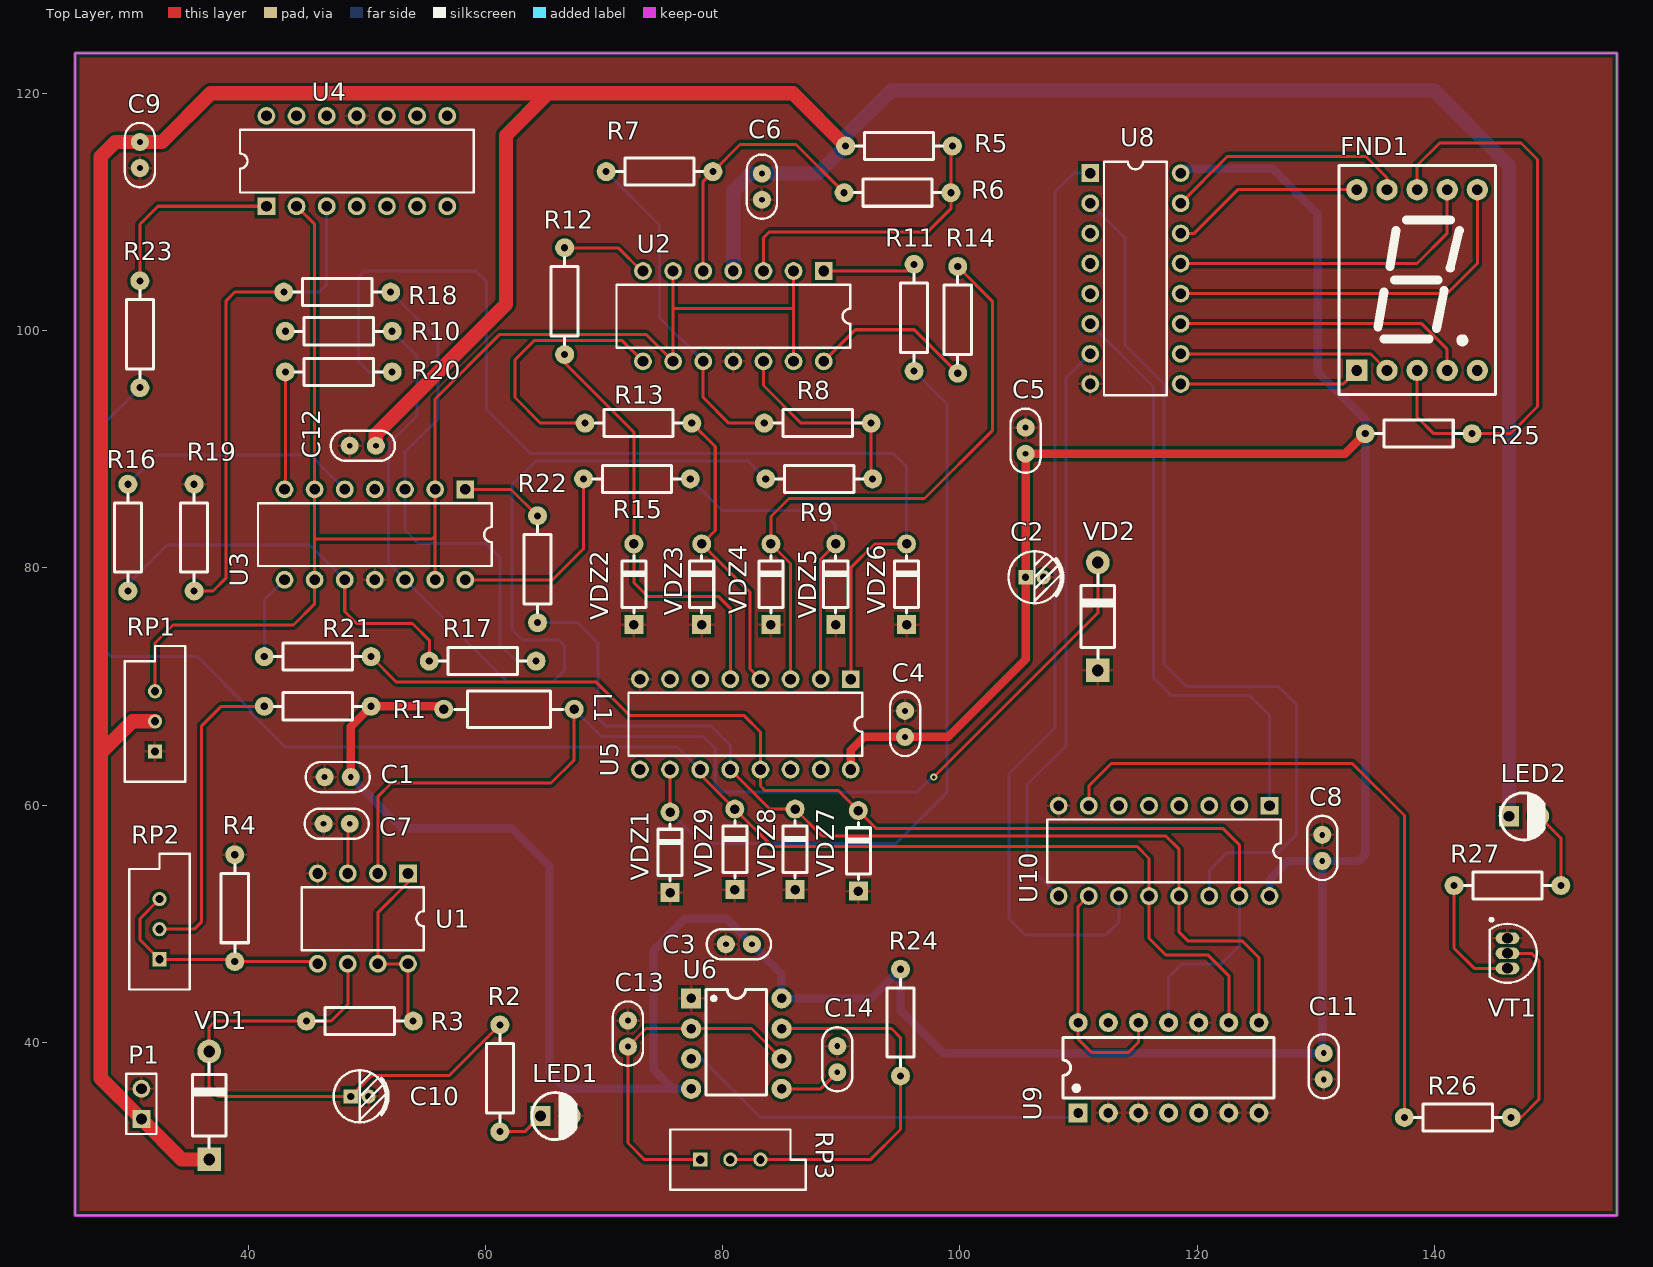
[diagram p0: Top Layer view]
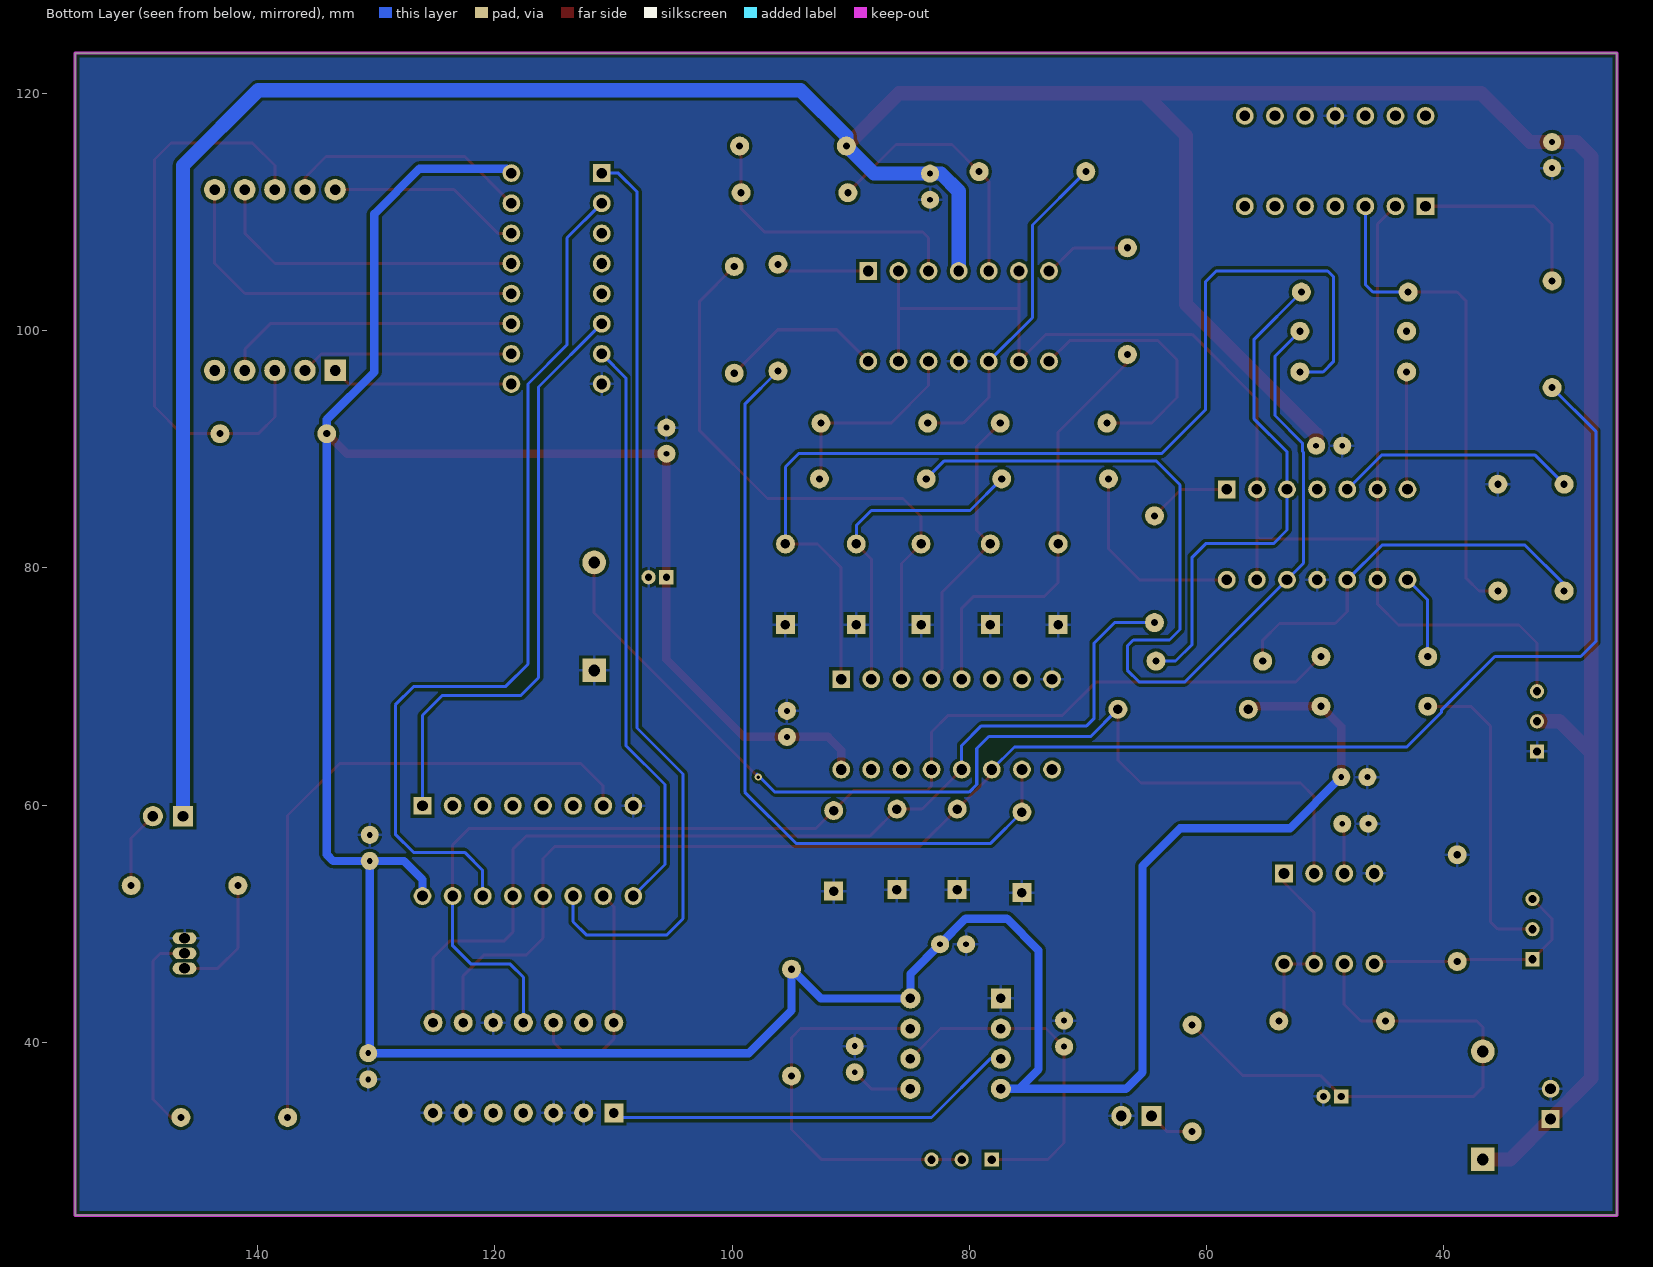
[diagram p1: Bottom Layer view, seen from below]
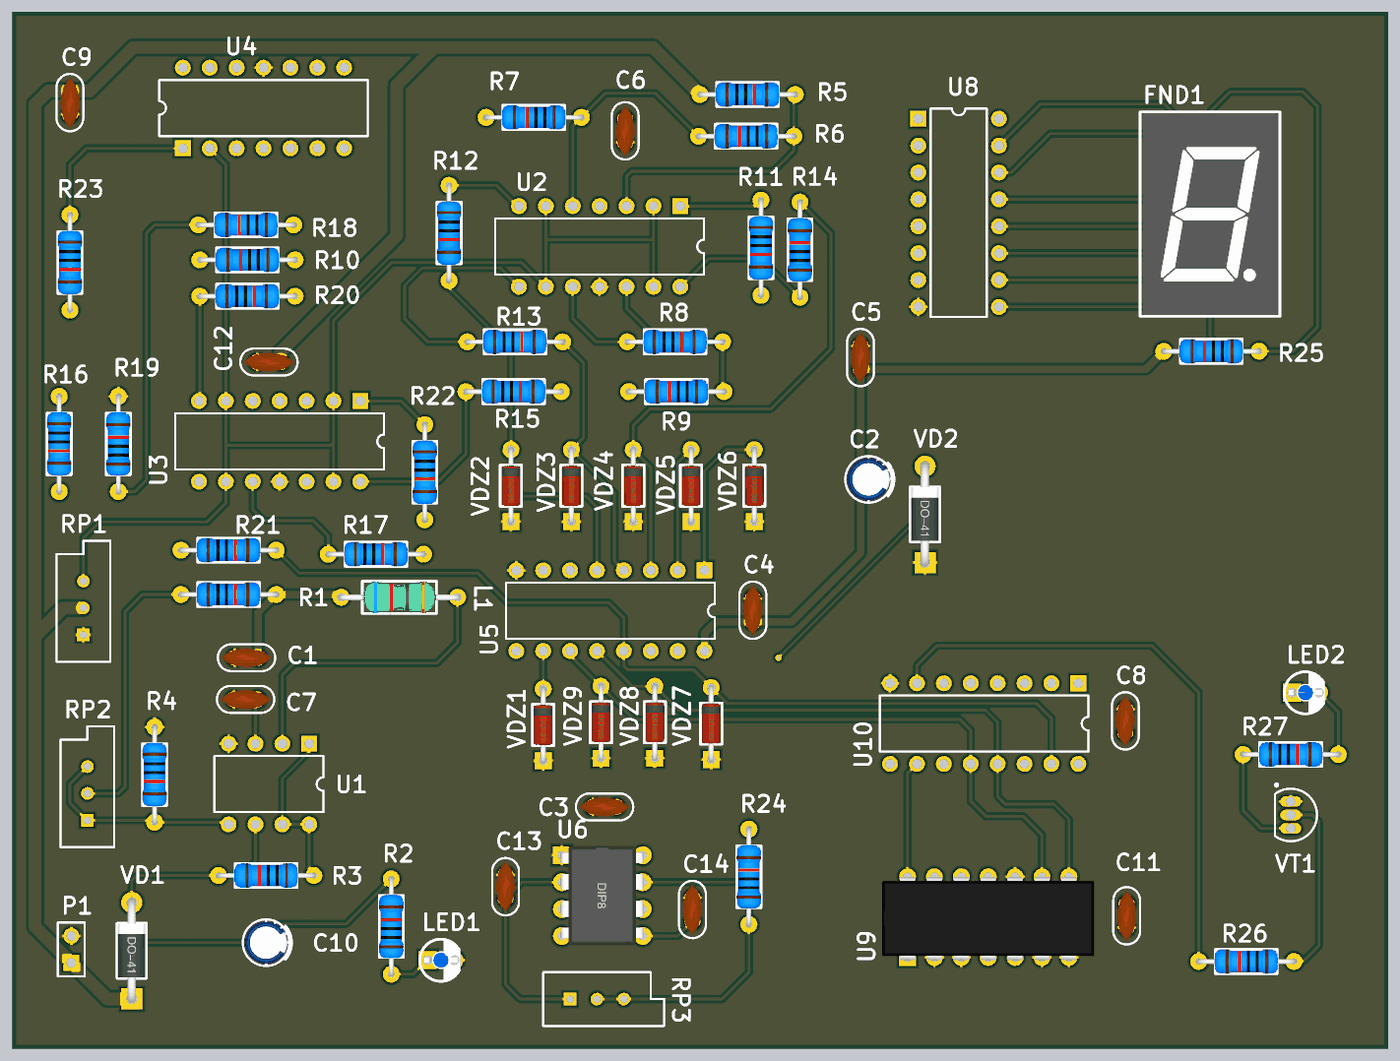
[diagram p2: 3D render of the assembled board from above, using the file's embedded part models]
# Altium PCB MISC80768.PcbDoc
Units mm, origin at the board's own origin, x right, y up, seen from the top; angles counter-clockwise.
Board outline 130 x 98 mm, 2 copper layers (Top Layer, Bottom Layer); 70 components, 65 nets, 254 pads, 1 vias.

## Layer stack, top to bottom (the 12.6 mil dielectric is the usual default, probably not edited)
Top Solder: solder mask 0.0102, Solder Resist, Dk 3.5
Top Layer: signal copper 0.0356
Dielectric 1: dielectric 0.32, FR-4, Dk 4.8
Bottom Layer: signal copper 0.0356
Bottom Solder: solder mask 0.0102, Solder Resist, Dk 3.5

## Board outline
25.4,25.4 25.4,123.4 155.4,123.4 155.4,25.4

## Design rules (kind name [scope] priority, off if disabled: settings)
Clearance [All] p1: gap=0.254
MinimumSolderMaskSliver [All] p1: minsoldermaskwidth=0
PolygonConnect [All] p1: connectstyle=Relief reliefconductorwidth=0.254 reliefentries=4 polygonreliefangle="90 Angle" airgapwidth=0.254
RoutingVias [All] p1: holewidth=0.711 width=1.27 viastyle="Through Hole" minholewidth=0.711 minwidth=1.27 maxholewidth=0.711 maxwidth=1.27
SilkToSilkClearance [All] p1: silktosilkclearance=0
SilkToSolderMaskClearance [IsPad] p1: minsilkscreentomaskgap=0 clearancetoexposedcopper=TRUE
SolderMaskExpansion [All] p1: expansion=0.102
Width [All] p1: maxlimit=2 minlimit=0.254 preferedwidth=0.254
27 further rules are at their usual default settings.

## Components (designator, comment, footprint, x,y, rotation, side; value= is the part's Value field where it differs from the comment)
C1 "104" "CC 2.2*5" 47.541,62.357 r180 top
C2 "470UF" "CAP 1.5*4*8" 106.299,79.205 r0 top
C3 "0.1uF" "CC 2.2*5" 81.364,48.26 r180 top
C4 "0.1uF" "CC 2.2*5" 95.377,66.845 r90 top
C5 "0.1uF" "CC 2.2*5" 105.537,90.721 r90 top
C6 "0.1uF" "CC 2.2*5" 83.312,112.141 r270 top
C7 "470PF" "CC 2.2*5" 47.455,58.42 r180 top
C8 "0.1uF" "CC 2.2*5" 130.556,56.388 r90 top
C9 "0.1uF" "CC 2.2*5" 30.861,114.808 r270 top
C10 "100UF" "CAP 1.5*4*8" 49.391,35.433 r0 top
C11 "0.1uF" "CC 2.2*5" 130.683,37.973 r270 top
C12 "0.1uF" "CC 2.2*5" 49.657,90.297 r180 top
C13 "0.1uF" "CC 2.2*5" 72.009,40.724 r90 top
C14 "0.1uF" "CC 2.2*5" 89.662,38.565 r90 top
FND1 "5011B" "SMG 0.5-1P" 138.557,104.267 r0 top
L1 "220uH" AL0307 61.976,68.072 r0 top
LED1 "red" "LED 3MM-B" 65.913,33.782 r0 top
LED2 "red" "LED 3MM-B" 147.574,59.055 r0 top
P1 "Header 2" HDR1X2 30.988,33.528 r90 top
R1 "3.3K" "RS 1/4W" 45.847,68.326 r0 top
R2 "2.2K" "RS 1/4W" 61.214,36.957 r90 top
R3 "0.5" "RS 1/4W" 49.403,41.783 r180 top
R4 "2.2K" "RS 1/4W" 38.862,51.308 r270 top
R5 "4.7K" "RS 1/4W" 94.869,115.57 r0 top
R6 "4.7K" "RS 1/4W" 94.742,111.633 r180 top
R7 "4.7K" "RS 1/4W" 74.676,113.411 r180 top
R8 "4.7K" "RS 1/4W" 88.011,92.202 r0 top
R9 "4.7K" "RS 1/4W" 88.138,87.503 r180 top
R10 "4.7K" "RS 1/4W" 47.625,99.949 r180 top
R11 "1K" "RS 1/4W" 96.139,101.092 r270 top
R12 "1K" "RS 1/4W" 66.675,102.489 r270 top
R13 "1K" "RS 1/4W" 72.898,92.202 r0 top
R14 "1K" "RS 1/4W" 99.822,100.91 r90 top
R15 "1K" "RS 1/4W" 72.771,87.503 r0 top
R16 "4.7K" "RS 1/4W" 29.845,82.55 r270 top
R17 "4.7K" "RS 1/4W" 59.762,72.136 r0 top
R18 "4.7K" "RS 1/4W" 47.498,103.251 r180 top
R19 "4.7K" "RS 1/4W" 35.433,82.55 r90 top
R20 "1K" "RS 1/4W" 47.625,96.52 r0 top
R21 "1K" "RS 1/4W" 45.847,72.517 r0 top
R22 "1K" "RS 1/4W" 64.389,79.883 r270 top
R23 "1K" "RS 1/4W" 30.861,99.695 r270 top
R24 "20K" "RS 1/4W" 94.996,41.656 r90 top
R25 "330" "RS 1/4W" 138.684,91.313 r180 top
R26 "4.7K" "RS 1/4W" 141.986,33.655 r180 top
R27 "1K" "RS 1/4W" 146.177,53.213 r0 top
RP1 "100K" VR5 32.131,67.056 r90 top
RP2 "5K" VR5 32.512,49.53 r90 top
RP3 "50K" VR5 80.645,30.099 r0 top
U1 "MC34063AP1" 626-05 49.657,50.419 r180 top
U2 "LM324AN" 646-06 80.899,101.219 r180 top
U3 "LM324AN" 646-06 50.673,82.804 r180 top
U4 "LM324AN" 646-06 49.149,114.3 r0 top
U5 "SN74LS147N" 648-08 81.915,66.802 r180 top
U6 "NE555" DIP8 81.153,39.878 r0 top
U8 "SN74LS47N" 648-08 114.808,104.394 r270 top
U9 "SN74LS90" DIP14 109.982,34.036 r90 top
U10 "SN74LS85N" 648-08 117.221,56.134 r180 top
VD1 "1N4007" DO-41 36.703,34.671 r90 top
VD2 "1N5819" DO-41 111.633,75.903 r90 top
VDZ1 "5.1V" DO-35 75.565,56.007 r90 top
VDZ2 "5.1V" DO-35 72.517,78.613 r90 top
VDZ3 "5.1V" DO-35 78.232,78.613 r90 top
VDZ4 "5.1V" DO-35 84.074,78.613 r90 top
VDZ5 "5.1V" DO-35 89.535,78.613 r90 top
VDZ6 "5.1V" DO-35 95.504,78.613 r90 top
VDZ7 "5.1V" DO-35 91.44,56.134 r90 top
VDZ8 "5.1V" DO-35 86.106,56.261 r90 top
VDZ9 "5.1V" DO-35 81.026,56.261 r90 top
VT1 "TP41" TO-92A 146.177,47.498 r180 top

## Footprints (in the part's own frame and the unit in brackets; to place one, negate y for a bottom-side part, rotate by r counter-clockwise, add the part's x,y. Pads: shape width x height; smd on the part's side, far side on the other; paste and mask are expansions set on the pad)
626-05 [mm] "DIP; 8 Leads; Row Spacing 7.62 mm; Pitch 2.54 mm"
  rect 1.5x1.5 hole 0.9: 1(-3.81,-3.81)
  round 1.5 hole 0.9: 2(-1.27,-3.81) 3(1.27,-3.81) 4(3.81,-3.81) 5(3.81,3.81) 6(1.27,3.81) 7(-1.27,3.81) 8(-3.81,3.81)
  silkscreen extent -5.15,-2.65 5.15,2.65
646-06 [mm] "DIP; 14 Leads; Row Spacing 7.62 mm; Pitch 2.54 mm"
  rect 1.5x1.5 hole 0.9: 1(-7.62,-3.81)
  round 1.5 hole 0.9: 2(-5.08,-3.81) 3(-2.54,-3.81) 4(0,-3.81) 5(2.54,-3.81) 6(5.08,-3.81) 7(7.62,-3.81) 8(7.62,3.81) 9(5.08,3.81) 10(2.54,3.81) 11(0,3.81) 12(-2.54,3.81) 13(-5.08,3.81) 14(-7.62,3.81)
  silkscreen extent -9.85,-2.65 9.85,2.65
648-08 [mm] "DIP; 16 Leads; Row Spacing 7.62 mm; Pitch 2.54 mm"
  rect 1.5x1.5 hole 0.9: 1(-8.89,-3.81)
  round 1.5 hole 0.9: 2(-6.35,-3.81) 3(-3.81,-3.81) 4(-1.27,-3.81) 5(1.27,-3.81) 6(3.81,-3.81) 7(6.35,-3.81) 8(8.89,-3.81) 9(8.89,3.81) 10(6.35,3.81) 11(3.81,3.81) 12(1.27,3.81) 13(-1.27,3.81) 14(-3.81,3.81) 15(-6.35,3.81) 16(-8.89,3.81)
  silkscreen extent -9.85,-2.65 9.85,2.65
AL0307 [mm] "11*3*7mm（脚距，直径，长度）"
  round 1.6 hole 0.8: 1(-5.5,0) 2(5.5,0)
  silkscreen extent -4.57,-1.52 4.57,1.52, body extent -5.78,-1.51 5.78,1.51, height 3.06
"CAP 1.5*4*8" [mm] "脚距1.5mm直径4mm高度8mm"
  rect 1.2x1.2 hole 0.6: 1(-0.75,0)
  round 1.2 hole 0.6: 2(0.75,0)
  silkscreen extent -2.2,-2.2 2.41,2.2, body extent -2,-2 2.02,2, height 8.04
"CC 2.2*5" [mm] "脚距2.2mm直径5mm"
  round 1.524 hole 0.5: 1(-1.1,0) 2(1.1,0)
  silkscreen extent -2.71,-1.27 2.71,1.27, body extent -2.4,-0.92 2.4,0.92, height 4.8
DIP8 [mm]
  rect 1.7x1.7 hole 0.8: 1(-3.81,3.81)
  round 1.7 hole 0.8: 2(-3.81,1.27) 3(-3.81,-1.27) 4(-3.81,-3.81) 5(3.81,-3.81) 6(3.81,-1.27) 7(3.81,1.27) 8(3.81,3.81)
  silkscreen extent -2.54,-4.32 2.54,4.57, body extent -3.94,-4.7 3.91,4.7, height 4.5
DIP14 [mm]
  rect 1.6x1.6 hole 0.813: 1(0,0)
  round 1.6 hole 0.813: 2(0,-2.54) 3(0,-5.08) 4(0,-7.62) 5(0,-10.16) 6(0,-12.7) 7(0,-15.24) 8(7.62,-15.24) 9(7.62,-12.7) 10(7.62,-10.16) 11(7.62,-7.62) 12(7.62,-5.08) 13(7.62,-2.54) 14(7.62,0)
  silkscreen extent 1.27,-16.51 6.35,1.27, body extent -0.25,-17.62 7.62,2.38, height 5.1
DO-35 [mm] "1.8*6.8mm(直径，脚距）"
  rect 1.6x1.6 hole 0.8: 1(-3.4,0)
  round 1.6 hole 0.8: 2(3.4,0)
  silkscreen extent -2.41,-1.02 2.41,1.02, body extent -3.65,-0.9 3.65,0.9, height 1.85
DO-41 [mm] "2.6*9.1mm(直径，脚距）"
  rect 2x2 hole 1: 1(-4.55,0)
  round 2 hole 1: 2(4.55,0)
  silkscreen extent -3.56,-1.4 3.56,1.4, body extent -4.92,-1.29 4.98,1.31, height 2.65
HDR1X2 [mm] "Connector; Header; 2 Position"
  rect 1.5x1.5 hole 0.9: 1(0,0)
  round 1.5 hole 0.9: 2(2.54,0)
  silkscreen extent -1.27,-1.27 3.81,1.27
"LED 3MM-B" [mm]
  rect 1.7x1.7 hole 0.9: 1(-1.27,0)
  round 1.7 hole 0.9: 2(1.27,0)
  silkscreen extent -2.01,-2 1.72,1.98, body extent -1.95,-1.95 1.64,1.95, height 5.55
"RS 1/4W" [mm] "直插色环电阻，脚距9mm，直径2.3mm"
  round 1.6 hole 0.6: 1(-4.5,0) 2(4.5,0)
  silkscreen extent -3.68,-1.14 3.68,1.14, body extent -4.72,-1.16 4.73,1.16, height 2.32
"SMG 0.5-1P" [mm] "12.7*19*8mm(长宽厚)"
  rect 1.8x1.8 hole 0.9: 1(-5.08,-7.62)
  round 1.8 hole 0.9: 2(-2.54,-7.62) 3(0,-7.62) 4(2.54,-7.62) 5(5.08,-7.62) 6(5.08,7.62) 7(2.54,7.62) 8(0,7.62) 9(-2.54,7.62) 10(-5.08,7.62)
  silkscreen extent -6.6,-9.65 6.6,9.65, body extent -6.35,-9.5 6.35,9.5, height 8
TO-92A [mm] "TO, Flat Index; 3 In-Line, Axial Leads; Body Dia. 4.5mm; Leads 0.51 x 0.48 mm (max)"
  oval 2x1 hole 0.9: 1(0,-1.27) 2(0,0) 3(0,1.27)
  silkscreen extent -2.48,-2.95 1.5,2.48, body extent -2.48,-2.5 1.5,2.5, height 6.86
VR5 [mm] "Thru-Hole; 3 Leads"
  rect 1.2x1.2 hole 0.7: 1(-2.54,0)
  round 1.2 hole 0.7: 2(0,0) 3(2.54,0)
  silkscreen extent -5.08,-2.54 6.35,2.54

## Part data
C1 C3 C4 C5 C6 C7 C8 C9 C11 C12 C13 C14: library part CC, "ceramic capacitor"
C2 C10: library part "Cap Pol2", "Polarized Capacitor (Axial)"
FND1: "0.5 inch 1-digit common-anode seven-segment display"
L1: library part L-AL, "color-band inductor"
LED1 LED2: library part LED-3MM, "3mm through-hole LED"
P1: "Header, 2-Pin"
R1 R2 R3 R4 R5 R6 R7 R8 R9 R10 R11 R12 R13 R14 R15 R16 R17 R18 R19 R20 R21 R22 R23 R24 R25 R26 R27: library part R-S, "color-band resistor"
RP1 RP2 RP3: library part RPot, "Potentiometer"
U1: "DC-to-DC Converter Control Circuit"
U2 U3 U4: "Quad Low-Power Operational Amplifier"
U5: "10-Line-to-4-Line Priority Encoder"
U6: library part NE555D, "General-Purpose Single Bipolar Timer"
U8: "BCD to 7-Segment Decoder/Driver"
U9: "DECADE DIV-BY-12 BIN CNT"
U10: "4-Bit Magnitude Comparator"
VD1: "rectifier diode"
VD2: library part 1N4007, "rectifier diode"
VDZ1 VDZ2 VDZ3 VDZ4 VDZ5 VDZ6 VDZ7 VDZ8 VDZ9: library part 1N4619, "3V/0.5W zener diode"
VT1: library part 2N3904, "NPN General Purpose Amplifier"

## Via types
v1: diameter 0.61, hole 0.305, Top Layer to Bottom Layer, 1 vias

## Nets (pads, with @x,y where several pads share a name; then routed paths per layer and width w, separated by ;. In a path a pad name is that pad's centre, name@x,y a point inside that pad or via, vN(x,y) a via of type N, cw(c..) or ccw(c..) an arc to the next point about the centre after c; other vN are vias at no path point)
+5V: C1.1 C2.1 C3.1 C4.1 C5.1 C8.1 C11.1 L1.1 R1.2 R24.2 R25.2 U5.16 U6.4 U6.8 U8.16 U10.16 | length 304.5
  Top Layer w0.7: C1.1 48.641,66.62 R1.2 56.222,68.326 L1.1 ; U5.16 90.805,64.643 91.907,65.745 C4.1 99.019,65.745 105.549,72.275 C2.1 105.549,89.609 C5.1 132.492,89.621 R25.2
  Bottom Layer w0.7: C1.1 52.959,58.039 62.23,58.039 65.405,54.864 65.405,37.465 66.802,36.068 75.819,36.068 ; U6.4 75.819,36.068 ; U8.16 118.999,113.665 126.365,113.665 130.175,109.855 130.175,96.52 134.184,92.511 R25.2 134.184,55.825 133.647,55.288 C8.1 ; U10.16 126.111,53.721 127.678,55.288 C8.1 ; 75.819,36.068 74.168,37.719 74.168,47.752 76.835,50.419 80.305,50.419 C3.1 84.963,45.761 U6.8 92.528,43.688 R24.2 94.996,42.672 98.595,39.073 C11.1 130.556,39.2 C8.1
+10V: C6.1 C9.1 C12.1 LED2.1 P1.1 R5.1 RP1.2 U2.4 VD1.1 | length 331.6
  Top Layer w1.2: RP1.2 30.226,67.056 27.559,64.389 ; VD1.1 34.395,30.121 P1.1 27.559,36.957 27.559,64.389 ; C12.1 50.757,91.27 61.722,102.235 61.722,116.459 65.278,120.015 ; R5.1 85.924,120.015 65.278,120.015 ; 27.559,64.389 27.559,114.681 28.786,115.908 C9.1 32.723,115.908 36.83,120.015 65.278,120.015
  Bottom Layer w1.2: U2.4 80.899,111.76 82.38,113.241 C6.1 88.04,113.241 R5.1 90.369,116.404 94.234,120.269 139.954,120.269 146.304,113.919 LED2.1
A: R10.2
CLK: U6.3 U9.1 | length 34.8
  Bottom Layer w0.254: U6.3 78.232,38.608 83.185,33.655 109.601,33.655 U9.1
D0: U9.12 U9.14 U10.10 | length 20
  Top Layer w0.254: U10.10 109.982,51.435 U9.14 109.982,40.259 111.125,39.116 114.173,39.116 115.062,40.005 U9.12
D1: R23.2 U5.11 U9.9 U10.12 VDZ9.2 | length 138.4
  Top Layer w0.254: U5.11 78.105,62.582 VDZ9.2 84.172,56.515 114.935,56.515 115.951,55.499 U10.12 115.951,48.768 117.348,47.371 120.904,47.371 122.682,45.593 U9.9
  Bottom Layer w0.254: R23.2 27.178,91.512 27.178,73.787 28.448,72.517 35.687,72.517 40.166,68.038 40.166,67.837 43.106,64.897 76.2,64.897 U5.11
D2: R22.2 U5.12 U9.8 U10.13 VDZ8.2 | length 87
  Top Layer w0.254: U5.12 83.976,59.661 VDZ8.2 88.363,57.404 117.348,57.404 118.491,56.261 U10.13 118.491,49.276 119.253,48.514 123.825,48.514 125.222,47.117 U9.8
  Bottom Layer w0.254: R22.2 67.746,75.383 69.469,73.66 69.469,67.31 70.104,66.675 78.994,66.675 80.645,65.024 U5.12
D3: R21.2 U5.13 U9.11 U10.15 VDZ7.2 | length 101.9
  Top Layer w0.254: R21.2 52.506,70.358 69.342,70.358 72.136,67.564 81.788,67.564 83.185,66.167 U5.13 83.185,61.595 83.566,61.214 89.76,61.214 VDZ7.2 92.935,58.039 122.174,58.039 123.571,56.642 U10.15
  Bottom Layer w0.254: U9.11 117.602,45.466 118.745,46.609 122.047,46.609 123.571,48.133 U10.15
D4: R20.2 U5.1 VDZ6.2 | length 91.4
  Top Layer w0.254: U5.1 90.805,80.01 92.808,82.013 VDZ6.2
  Bottom Layer w0.254: R20.2 50.165,96.52 49.276,97.409 49.276,104.521 49.784,105.029 59.182,105.029 60.071,104.14 60.071,93.345 63.754,89.662 94.361,89.662 95.504,88.519 VDZ6.2
D5: R15.2 U5.2 VDZ5.2 | length 27.4
  Top Layer w0.254: U5.2 88.265,80.743 VDZ5.2
  Bottom Layer w0.254: R15.2 79.938,84.836 88.265,84.836 89.535,83.566 VDZ5.2
D6: R14.2 U5.3 VDZ4.2 | length 51.1
  Top Layer w0.254: U5.3 85.725,80.362 VDZ4.2 84.074,84.328 85.598,85.852 97.028,85.852 102.743,91.567 102.743,102.489 R14.2
D7: R13.2 U5.4 VDZ3.2 | length 24.9
  Top Layer w0.254: R13.2 79.375,90.225 79.375,83.156 VDZ3.2 82.296,77.949 82.296,71.501 U5.4
D8: R12.2 U5.5 VDZ2.2 | length 36.7
  Top Layer w0.254: R12.2 66.675,97.282 72.517,91.44 VDZ2.2 72.517,78.74 73.66,77.597 79.629,77.597 80.645,76.581 U5.5
D9: R11.2 U5.10 VDZ1.2 | length 66.5
  Top Layer w0.254: VDZ1.2 U5.10
  Bottom Layer w0.254: VDZ1.2 78.203,56.769 94.615,56.769 98.933,61.087 98.933,93.798 R11.2
DQ0: U8.7 U10.9 | length 49
  Bottom Layer w0.254: U10.9 105.664,54.991 105.664,61.722 108.966,65.024 108.966,96.012 U8.7
DQ1: U8.1 U10.11 | length 79
  Bottom Layer w0.254: U8.1 109.601,113.284 108.03,111.713 108.03,66.501 104.14,62.611 104.14,50.419 105.537,49.022 112.268,49.022 113.411,50.165 U10.11
DQ2: U8.2 U10.14 | length 75.7
  Bottom Layer w0.254: U8.2 113.919,107.823 113.919,98.806 117.221,95.504 117.221,71.882 119.126,69.977 126.873,69.977 128.397,68.453 128.397,57.531 126.873,56.007 122.555,56.007 121.031,54.483 U10.14
DQ3: U8.6 U10.1 | length 50.8
  Bottom Layer w0.254: U8.6 116.332,95.25 116.332,70.739 117.856,69.215 124.46,69.215 126.111,67.564 U10.1
GND: C1.2 C2.2 C3.2 C4.2 C5.2 C6.2 C7.2 C8.2 C9.2 C10.2 C11.2 C12.2 C13.2 C14.2 LED1.2 P1.2 R4.1 R19.2 RP1.1 U1.4 U2.11 U3.11 U4.11 U5.8 U6.1 U8.8 U9.2 U9.3 U9.6 U9.7 U9.10 U10.8 VD2.1 VDZ1.1 VDZ2.1 VDZ3.1 VDZ4.1 VDZ5.1 VDZ6.1 VDZ7.1 VDZ8.1 VDZ9.1 VT1.1
NetC7_1: C7.1 U1.3 | length 4.3
  Top Layer w0.254: U1.3 48.387,58.252 C7.1
NetC10_1: C10.1 R2.2 R3.2 U1.6 VD1.2 | length 48.3
  Top Layer w0.254: U1.6 48.387,43.18 46.99,41.783 R3.2 37.211,41.783 36.703,41.275 VD1.2 36.703,36.195 37.465,35.433 C10.1 50.419,37.211 56.968,37.211 R2.2
NetC13_1: C13.1 RP3.1 U6.2 U6.6 | length 29.4
  Top Layer w0.254: RP3.1 73.406,30.099 72.009,31.496 C13.1 73.533,41.148 U6.2 82.423,41.148 U6.6
NetC14_1: C14.1 U6.5 | length 5.3
  Top Layer w0.254: U6.5 88.265,36.068 C14.1
NetFND1_1: FND1.1 U8.9 | length 15.3
  Top Layer w0.254: U8.9 132.334,95.504 FND1.1
NetFND1_2: FND1.2 U8.10 | length 18
  Top Layer w0.254: U8.10 134.62,98.044 FND1.2
NetFND1_3: FND1.3 FND1.8 R25.1 | length 50
  Top Layer w0.254: FND1.3 138.557,92.71 139.954,91.313 R25.1 146.431,91.313 148.717,93.599 148.717,114.427 147.32,115.824 140.462,115.824 138.557,113.919 FND1.8
NetFND1_4: FND1.4 U8.11 | length 25.2
  Top Layer w0.254: U8.11 138.938,100.584 141.097,98.425 FND1.4
NetFND1_6: FND1.6 U8.12 | length 32.3
  Top Layer w0.254: U8.12 141.097,103.124 143.637,105.664 FND1.6
NetFND1_7: FND1.7 U8.13 | length 27.2
  Top Layer w0.254: U8.13 138.557,105.664 141.097,108.204 FND1.7
NetFND1_9: FND1.9 U8.15 | length 20.8
  Top Layer w0.254: U8.15 122.555,114.681 134.239,114.681 136.017,112.903 FND1.9
NetFND1_10: FND1.10 U8.14 | length 16.4
  Top Layer w0.254: U8.14 119.761,108.204 123.444,111.887 FND1.10
NetL1_2: L1.2 U1.2 VD2.2 | length 88.2
  Top Layer w0.254: U1.2 50.927,60.706 52.07,61.849 65.532,61.849 67.476,63.793 L1.2 ; v1(97.79,62.357) 111.633,76.2 VD2.2
  Bottom Layer w0.254: L1.2 69.762,65.786 78.359,65.786 79.375,64.77 79.375,61.722 80.01,61.087 96.393,61.087 v1@97.917,62.611
NetLED1_1: LED1.1 R2.1 | length 4
  Top Layer w0.254: R2.1 63.318,32.457 LED1.1
NetLED2_2: LED2.2 R27.2 | length 6.6
  Top Layer w0.254: LED2.2 150.677,57.222 R27.2
NetR1_1: R1.1 RP2.2 | length 26.3
  Top Layer w0.254: RP2.2 35.433,49.53 36.068,50.165 36.068,66.675 37.719,68.326 R1.1
NetR3_1: R3.1 U1.1 U1.7 U1.8 | length 16.2
  Top Layer w0.254: U1.1 53.467,53.467 50.927,50.927 U1.7 U1.8 53.467,42.219 R3.1
NetR4_2: R4.2 RP2.1 RP2.3 U1.5 | length 19.9
  Top Layer w0.254: RP2.3 30.861,50.419 30.861,48.641 RP2.1 38.68,46.99 R4.2 45.648,46.808 U1.5
NetR5_2: R5.2 R6.1 U2.3 | length 25
  Top Layer w0.254: U2.3 83.439,107.823 83.947,108.331 97.282,108.331 99.242,110.291 R6.1 99.242,115.443 R5.2
NetR6_2: R6.2 R7.1 U2.5 | length 22.4
  Top Layer w0.254: U2.5 78.359,112.594 R7.1 81.462,115.697 86.178,115.697 R6.2
NetR7_2: R7.2 R8.1 U2.10 | length 28.5
  Top Layer w0.254: U2.10 78.359,94.361 80.518,92.202 R8.1
  Bottom Layer w0.254: R7.2 74.676,108.911 74.676,101.092 U2.10
NetR8_2: R8.2 R9.1 U2.12 | length 17.2
  Top Layer w0.254: U2.12 83.439,95.377 86.614,92.202 R8.2 92.511,87.63 R9.1
NetR9_2: R9.2 R10.1 U3.12 | length 83
  Bottom Layer w0.254: R10.1 54.229,97.845 54.229,92.837 51.9,90.508 51.9,89.824 51.816,89.74 51.816,80.391 U3.12 61.849,70.358 65.659,70.358 66.675,71.374 66.675,73.406 66.167,73.914 63.119,73.914 62.23,74.803 62.23,86.995 64.262,89.027 82.114,89.027 R9.2
NetR11_1: R11.1 U2.1 | length 7.9
  Top Layer w0.254: U2.1 95.576,105.029 R11.1
NetR12_1: R12.1 U2.7 | length 7.4
  Top Layer w0.254: R12.1 71.192,106.989 73.152,105.029 U2.7
NetR13_1: R13.1 U2.8 | length 22.2
  Top Layer w0.254: R13.1 64.643,92.202 62.484,94.361 62.484,97.536 64.135,99.187 71.501,99.187 U2.8
NetR14_1: R14.1 U2.14 | length 13.9
  Top Layer w0.254: U2.14 91.186,100.076 96.156,100.076 R14.1
NetR15_1: R15.1 U3.14 | length 17
  Top Layer w0.254: U3.14 65.659,78.994 68.271,81.606 R15.1
NetR16_1: R16.1 U3.5 | length 20.5
  Bottom Layer w0.254: R16.1 32.33,89.535 45.212,89.535 U3.5
NetR16_2: R16.2 R17.1 U3.10 | length 34
  Top Layer w0.254: U3.10 48.133,76.327 49.149,75.311 53.848,75.311 55.262,73.897 R17.1
  Bottom Layer w0.254: R16.2 29.845,78.613 33.147,81.915 45.212,81.915 U3.10
NetR17_2: R17.2 R18.1 U3.3 | length 42.8
  Bottom Layer w0.254: R18.1 56.007,99.242 56.007,92.583 53.213,89.789 U3.3 53.213,83.185 54.356,82.042 60.071,82.042 61.214,80.899 61.214,73.533 62.611,72.136 R17.2
NetR18_2: R18.2 R19.1 U4.3 | length 42.2
  Top Layer w0.254: R19.1 37.029,78.05 38.1,79.121 38.1,102.489 38.862,103.251 R18.2
  Bottom Layer w0.254: R18.2 45.974,103.251 46.609,103.886 U4.3
NetR20_1: R20.1 U3.7 | length 9.9
  Top Layer w0.254: U3.7 43.125,86.686 R20.1
NetR21_1: R21.1 U3.8 | length 7.2
  Bottom Layer w0.254: R21.1 41.347,77.288 U3.8
NetR22_1: R22.1 U3.1 | length 7
  Top Layer w0.254: U3.1 62.158,86.614 R22.1
NetR23_1: R23.1 U4.1 | length 16.1
  Top Layer w0.254: R23.1 30.861,108.966 32.385,110.49 U4.1
NetR24_1: R24.1 RP3.2 RP3.3 U6.7 | length 33.5
  Top Layer w0.254: RP3.2 RP3.3 92.456,30.099 94.996,32.639 R24.1 94.996,40.386 94.234,41.148 U6.7
NetR26_1: R26.1 VT1.2 | length 17.6
  Top Layer w0.254: VT1.2 148.209,47.498 148.844,46.863 148.844,35.179 147.32,33.655 R26.1
NetR27_1: R27.1 VT1.3 | length 10.5
  Top Layer w0.254: R27.1 141.677,47.934 143.383,46.228 VT1.3
NetU5_6: U5.6
NetU5_7: U5.7
NetU5_9: U5.9
NetU5_14: U5.14
PWM: R26.2 U10.7 | length 56.3
  Top Layer w0.254: U10.7 110.871,61.595 112.776,63.5 133.096,63.5 137.486,59.11 R26.2
VCC: U9.5
VR: RP1.3 U2.2 U2.6 U2.9 U2.13 U3.2 U3.6 U3.9 U3.13 U4.2 | length 127.3
  Top Layer w0.254: RP1.3 32.131,73.66 33.655,75.184 43.815,75.184 45.593,76.962 U3.9 45.593,82.423 ; U4.2 45.593,108.966 U3.6 45.593,82.423 ; U3.13 55.753,82.677 ; U2.6 75.819,101.854 ; U2.13 85.979,101.981 ; U2.2 85.979,101.981 ; 45.593,82.423 55.499,82.423 55.753,82.677 ; 55.753,82.677 U3.2 55.753,94.234 61.214,99.695 73.533,99.695 U2.9 75.819,101.854 ; 75.819,101.854 85.852,101.854 85.979,101.981
pads on no net: FND1.5 U3.4 U4.4 U4.5 U4.6 U4.7 U4.8 U4.9 U4.10 U4.12 U4.13 U4.14 U5.15 U8.3 U8.4 U8.5 U9.4 U9.13 U10.2 U10.3 U10.4 U10.5 U10.6

## Polygon pours and split planes (outlines as drawn)
GND on Bottom Layer "D" (solid, remove dead copper, pour order 0): 18.669,127.508 18.923,127.762 161.036,127.762 161.036,18.288 161.925,17.399 159.766,19.558 7.493,19.558
GND on Top Layer "D" (solid, remove dead copper, pour order 2): 13.208,130.683 157.099,130.683 157.48,131.064 160.782,127.762 160.782,26.035 160.782,20.447 158.877,18.542 155.575,15.24 17.78,15.24

## Keep-outs
Keep-Out Layer:
  the board outline again, w0.254